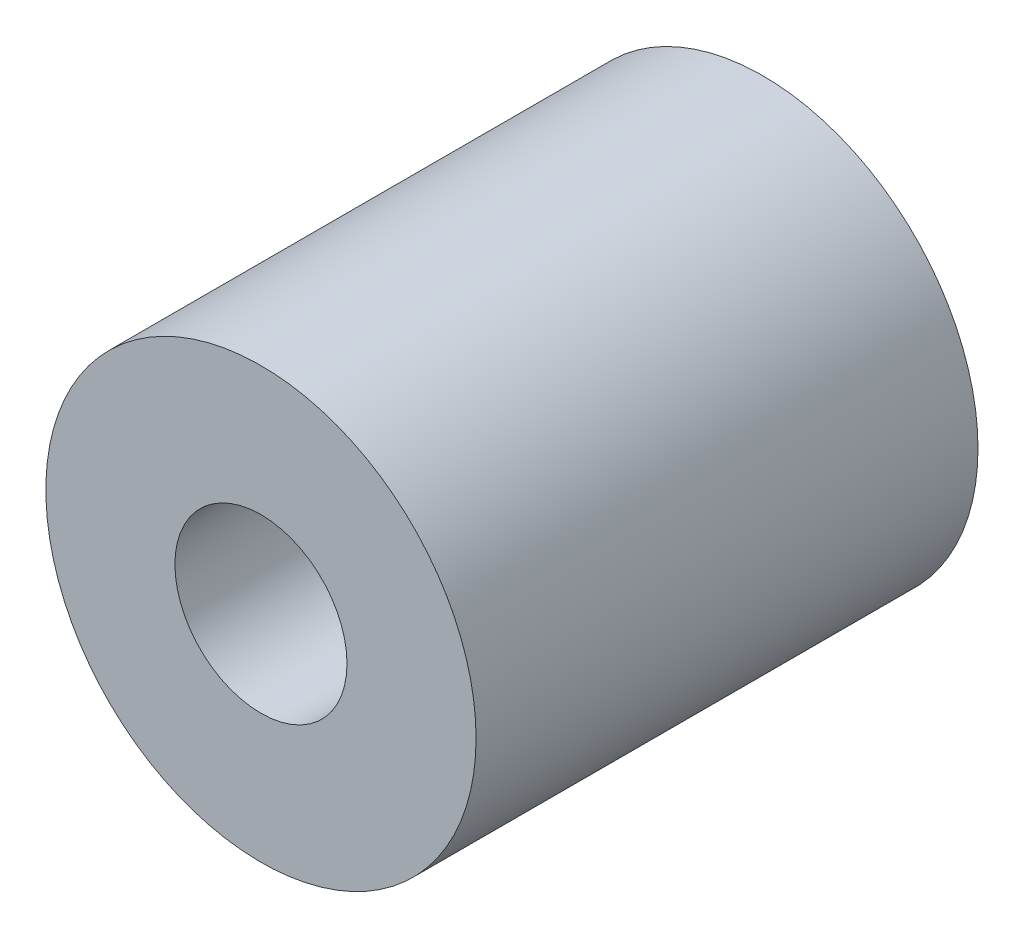
from build123d import *

# Parameters (mm, degrees)
SKETCH_1_R          = 15
EXTRUDE_1_DEPTH     = 35
SKETCH_2_R          = 6
CUT_EXTRUDE_1_DEPTH = 17.5
SKETCH_3_R          = 8
CUT_EXTRUDE_2_DEPTH = 17.5


with BuildPart() as part:
    # 草图1 → 凸台-拉伸1 (new body)
    with BuildSketch(Plane.XY):
        Circle(SKETCH_1_R)
    extrude(amount=EXTRUDE_1_DEPTH)

    # 草图2 → 切除-拉伸1 (cut)
    with BuildSketch(Plane.XY.offset(35)):
        Circle(SKETCH_2_R)
    extrude(amount=-CUT_EXTRUDE_1_DEPTH, mode=Mode.SUBTRACT)

    # 草图3 → 切除-拉伸2 (cut)
    with BuildSketch(Plane(origin=(0, 0, 0), x_dir=(-1, 0, 0), z_dir=(0, 0, -1))):
        Circle(SKETCH_3_R)
    extrude(amount=-CUT_EXTRUDE_2_DEPTH, mode=Mode.SUBTRACT)


solid = part.part
